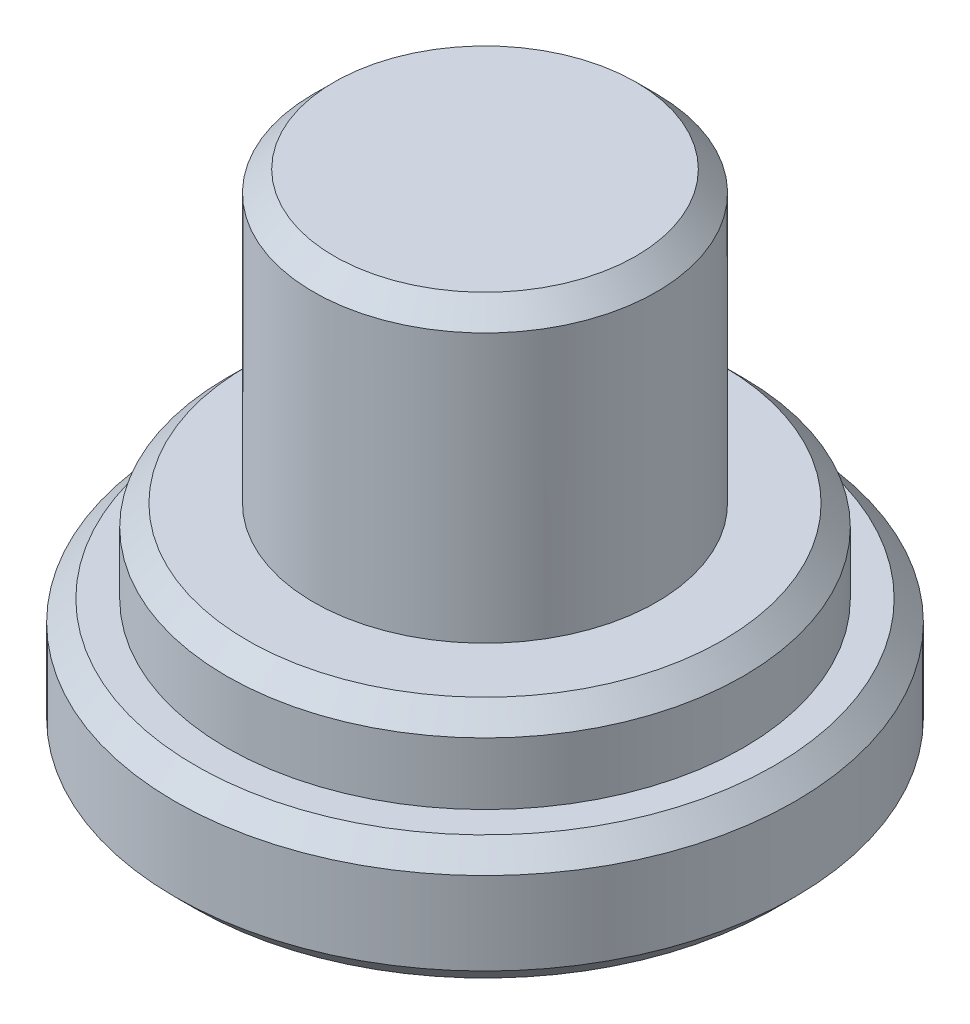
from build123d import *

# Parameters (mm, degrees)
CHAMFER1_SIZE = 0.5


with BuildPart() as part:
    # Sketch1 → Revolve1 (revolve)
    with BuildSketch(Plane.XY, mode=Mode.PRIVATE) as revolve1_sk:
        Polygon((154.87840727, -569.505265962), (152.77840727, -569.505265962), (152.77840727, -562.505265962), (148.62840727, -562.505265962), (148.62840727, -574.505265962), (156.12840727, -574.505265962), (156.12840727, -571.505265962), (154.87840727, -571.505265962), align=None)
    revolve(revolve1_sk.sketch.rotate(Axis((148.62840727, -560.805265962, 0), (0, -1, 0)), 180), axis=Axis((148.62840727, -560.805265962, 0), (0, -1, 0)))

    # Chamfer1
    chamfer1_edges = [part.edges().sort_by_distance(p)[0] for p in [
        (154.87840727, -569.505265962, 0),
        (156.12840727, -571.505265962, 0),
        (156.12840727, -574.505265962, 0),
        (152.77840727, -562.505265962, 0),
    ]]
    chamfer(chamfer1_edges, length=CHAMFER1_SIZE)


solid = part.part
